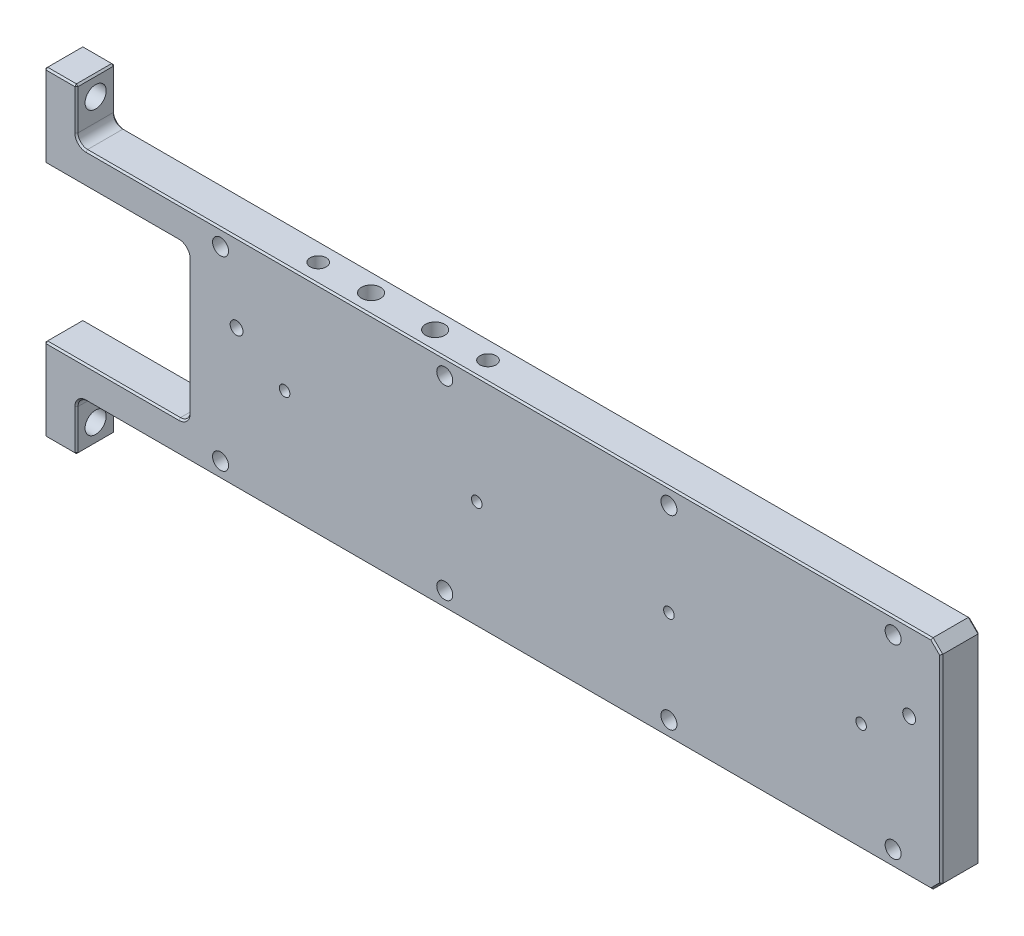
SolidWorks part; units mm, degrees
material "#45(1.1191)"
ref_plane "前视基准面" through (0, 0, 0) normal (0, 0, 1) x (1, 0, 0)
ref_plane "上视基准面" through (0, 0, 0) normal (0, 1, 0) x (1, 0, 0)
ref_plane "右视基准面" through (0, 0, 0) normal (1, 0, 0) x (0, 0, -1)
sketch "草图1" plane through (0, 0, 0) normal (0, 0, 1) x (1, 0, 0)
  line L1 (-140, -34) -> (140, -34)
  line L2 (-140, -34) -> (-140, 34)
  line L3 (-140, 34) -> (140, 34)
  line L4 (140, -34) -> (140, 34)
  line L5 (-140, -34) -> (140, 34) construction
  line L6 (-140, 34) -> (140, -34) construction
  point P0 (0, 0)
  dimension "D1" = 280
  dimension "D2" = 68
extrude "凸台-拉伸1" add sketch "草图1" along normal mid plane 12
sketch "草图2" plane through (0, 0, -6) normal (0, 0, -1) x (-1, 0, 0)
  line L0 (-140, 0) -> (140, 0) construction
  line L1 (95, -24) -> (140, -24)
  line L2 (95, -24) -> (95, 24)
  line L3 (95, 24) -> (140, 24)
  line L4 (140, -24) -> (140, 24)
  line L5 (-140, -34) -> (-140, 34) construction
  line L6 (140, 34) -> (140, -34) construction
  dimension "D1" = 48
  dimension "D2" = 45
extrude "切除-拉伸1" cut sketch "草图2" against normal blind 25
fillet "圆角1" radius 3 2 edges at (-95, -24, 0) (-95, 24, 0)
sketch "草图3" plane through (-140, 0, 0) normal (-1, 0, 0) x (0, 0, 1)
  line L0 (6, 0) -> (-6, 0) construction
  line L1 (6, 21) -> (6, -21) construction
  line L2 (-6, 21) -> (-6, -21) construction
  line L3 (0, 34) -> (0, -34) construction
  line L4 (6, 34) -> (-6, 34) construction
  line L5 (6, -34) -> (-6, -34) construction
  line L6 (-6, -24) -> (-6, -34) construction
  line L7 (6, -34) -> (-6, -34)
  line L8 (6, -34) -> (6, -50)
  line L9 (6, -50) -> (-6, -50)
  line L10 (-6, -34) -> (-6, -50)
  line L11 (-6, 34) -> (-6, 50)
  line L12 (6, 50) -> (-6, 50)
  line L13 (6, 34) -> (6, 50)
  line L14 (6, 34) -> (-6, 34)
  dimension "D1" = 16
extrude "凸台-拉伸2" add sketch "草图3" against normal blind 10
fillet "圆角2" radius 3 2 edges at (-130, 34, 0) (-130, -34, 0)
sketch "草图4" plane through (-130, 0, 0) normal (1, 0, 0) x (0, 0, -1)
  line L0 (0, -50) -> (0, 50) construction
  line L1 (6, -50) -> (-6, -50) construction
  line L2 (-6, 50) -> (6, 50) construction
  line L4 (-6, 0) -> (6, 0) construction
  line L5 (-6, -34) -> (-6, 34) construction
  line L6 (6, -34) -> (6, 34) construction
  point P0 (0, -44)
  point P18 (0, 44)
  dimension "D1" = 6
hole_wizard "M6 间隙孔1" positions "草图4" profile "草图5" hole size "M6" standard "ISO" end condition through all
sketch "草图5" plane through (-130, -44, 0) normal (0, 1, 0) x (0, 0, -1)
  line L0 (0, 0) -> (0, 10)
  line L1 (0, 10) -> (3.3, 10)
  line L2 (3.3, 10) -> (3.3, 0)
  line L5 (3.3, 0) -> (0, 0)
  line L11 (0, -6.35) -> (0, 107.95) construction
  dimension "通孔孔直径" = 6.6
  dimension "通孔孔深度" = 10
sketch "草图6" plane through (-140, 0, 0) normal (-1, 0, 0) x (0, 0, 1)
  line L0 (6, 0) -> (-6, 0) construction
  line L1 (6, 21) -> (6, -21) construction
  line L2 (-6, 21) -> (-6, -21) construction
  line L4 (0, 50) -> (0, -50) construction
  line L5 (6, 50) -> (-6, 50) construction
  line L6 (-6, -50) -> (6, -50) construction
  point P0 (0, 32.5)
  point P20 (0, -32.5)
  dimension "D1" = 65
hole_wizard "Ø6.0mm 暗销孔1" positions "草图6" profile "草图7" hole size "Ø6.0" standard "ISO"
sketch "草图7" plane through (-140, 32.5, 0) normal (0, 1, 0) x (0, 0, 1)
  line L0 (0, 0) -> (0, 11.8026)
  line L1 (0, 11.8026) -> (3, 10)
  line L2 (3, 10) -> (3, 0)
  line L5 (3, 0) -> (0, 0)
  line L10 (0, 11.8026) -> (-3, 10) construction
  line L11 (0, -6.35) -> (0, 107.95) construction
  dimension "孔直径" = 6
  dimension "孔深度" = 10
  dimension "导头角度" = 118
chamfer "倒角1" distance 3 angle 45 2 edges at (140, 34, 0) (140, -34, 0)
chamfer "倒角2" distance 0.5 angle 45 42 edges at (-119, 24, -6) (-119, 24, 6) (-119, -24, 6) (-119, -24, -6) (-95.8787, 23.1213, 6) (-95.8787, 23.1213, -6) (-95.8787, -23.1213, 6) (-95.8787, -23.1213, -6) (-95, 0, -6) (-95, 0, 6) (-135, -50, 6) (-130, -50, 0) (-135, -50, -6) (-140, -50, 0) (-140, -37, 6) (-140, -37, -6) (-140, -24, 0) (-135, 50, -6) (-130, 50, 0) (-135, 50, 6) (-140, 50, 0) (-140, 37, 6) (-140, 37, -6) (-140, 24, 0) (-130, 43.5, 6) (-130, -43.5, 6) (-129.1213, 34.8787, -6) (-129.1213, 34.8787, 6) (-129.1213, -34.8787, 6) (-129.1213, -34.8787, -6) (5, 34, 6) (5, 34, -6) (138.5, 32.5, 6) (138.5, 32.5, -6) (140, 0, -6) (140, 0, 6) (138.5, -32.5, 6) (138.5, -32.5, -6) (5, -34, -6) (5, -34, 6) (-130, 43.5, -6) (-130, -43.5, -6)
sketch "草图16" plane through (0, 0, -6) normal (0, 0, -1) x (-1, 0, 0)
  point P0 (-125, 29)
  point P3 (-125, -29)
  point P6 (-55, 29)
  point P9 (-55, -29)
  point P12 (15, 29)
  point P15 (15, -29)
  point P18 (85, 29)
  point P21 (85, -29)
hole_wizard "M6 螺纹孔3" positions "草图16" profile "草图17" tap size "M6" standard "ISO" end condition through all
sketch "草图17" plane through (125, 29, -6) normal (1, 0, 0) x (0, 1, 0)
  line L0 (0, 0) -> (0, 12)
  line L1 (0, 12) -> (2.5, 12)
  line L2 (2.5, 12) -> (2.5, 0)
  line L5 (2.5, 0) -> (0, 0)
  line L11 (0, -6.35) -> (0, 107.95) construction
  dimension "通孔螺纹孔钻头直径" = 5
  dimension "通孔螺纹孔钻头深度" = 12
cosmetic thread "孔螺蚊线14" parameters "D2"=6
cosmetic thread "孔螺蚊线15" parameters "D2"=6
cosmetic thread "孔螺蚊线16" parameters "D2"=6
cosmetic thread "孔螺蚊线17" parameters "D2"=6
cosmetic thread "孔螺蚊线18" parameters "D2"=6
cosmetic thread "孔螺蚊线19" parameters "D2"=6
cosmetic thread "孔螺蚊线22" parameters "D2"=6
cosmetic thread "孔螺蚊线23" parameters "D2"=6
sketch "草图18" plane through (0, 34, 0) normal (0, 1, 0) x (1, 0, 0)
  point P0 (-24, 0)
  point P3 (-44, 0)
hole_wizard "Ø6.0mm 暗销孔2" positions "草图18" profile "草图19" hole size "Ø6.0" standard "ISO"
sketch "草图19" plane through (-24, 34, 0) normal (1, 0, 0) x (0, 0, 1)
  line L0 (0, 0) -> (0, 7.8026)
  line L1 (0, 7.8026) -> (3, 6)
  line L2 (3, 6) -> (3, 0)
  line L5 (3, 0) -> (0, 0)
  line L10 (0, 7.8026) -> (-3, 6) construction
  line L11 (0, -6.35) -> (0, 107.95) construction
  dimension "孔直径" = 6
  dimension "孔深度" = 6
  dimension "导头角度" = 118
sketch "草图20" plane through (0, 34, 0) normal (0, 1, 0) x (1, 0, 0)
  point P0 (-7.5, 0)
  point P3 (-60.5, 0)
hole_wizard "M6 螺纹孔4" positions "草图20" profile "草图21" tap size "M6" standard "ISO"
sketch "草图21" plane through (-7.5, 34, 0) normal (1, 0, 0) x (0, 0, 1)
  line L0 (0, 0) -> (0, 16.5022)
  line L1 (0, 16.5022) -> (2.5, 15)
  line L2 (2.5, 15) -> (2.5, 0)
  line L5 (2.5, 0) -> (0, 0)
  line L10 (0, 16.5022) -> (-2.5, 15) construction
  line L11 (0, -6.35) -> (0, 107.95) construction
  dimension "螺纹孔钻头直径" = 5
  dimension "螺纹孔钻头深度" = 15
  dimension "导头角度" = 118
cosmetic thread "孔螺蚊线24" parameters "D1"=12, "D2"=6
cosmetic thread "孔螺蚊线25" parameters "D1"=12, "D2"=6
hole_wizard "M4 螺纹孔1" positions "草图23" profile "草图22" tap size "M4" standard "ISO" end condition through all
sketch "草图23" plane through (0, 0, 6) normal (0, 0, 1) x (1, 0, 0)
  circle A0 centre (115, 0) radius 2.25 construction
  circle A1 centre (55, 0) radius 2.25 construction
  circle A2 centre (-65, 0) radius 2.25 construction
  circle A3 centre (-5, 0) radius 2.25 construction
  point P1 (115, 0)
  point P4 (55, 0)
  point P7 (-65, 0)
  point P10 (-5, 0)
sketch "草图22" plane through (115, 0, 6) normal (1, 0, 0) x (0, -1, 0)
  line L0 (0, 0) -> (0, 12)
  line L1 (0, 12) -> (1.65, 12)
  line L2 (1.65, 12) -> (1.65, 0)
  line L5 (1.65, 0) -> (0, 0)
  line L11 (0, -6.35) -> (0, 107.95) construction
  dimension "通孔螺纹孔钻头直径" = 3.3
  dimension "通孔螺纹孔钻头深度" = 12
cosmetic thread "孔螺蚊线26" parameters "D2"=4
cosmetic thread "孔螺蚊线27" parameters "D2"=4
cosmetic thread "孔螺蚊线28" parameters "D2"=4
cosmetic thread "孔螺蚊线29" parameters "D2"=4
hole_wizard "Ø4.0 mm 暗销孔1" positions "草图25" profile "草图24" hole size "Ø4.0" standard "ISO"
sketch "草图25" plane through (0, 0, 6) normal (0, 0, 1) x (1, 0, 0)
  line L0 (135, 7.5) -> (-85, 7.5) construction
  point P1 (-80, 9.5)
  point P5 (130, 9.5)
  dimension "D1" = 2
  dimension "D2" = 5.3852
  dimension "D3" = 2
  dimension "D4" = 5.3852
sketch "草图24" plane through (-80, 9.5, 6) normal (1, 0, 0) x (0, -1, 0)
  line L0 (0, 0) -> (0, 5)
  line L1 (0, 5) -> (2, 5)
  line L2 (2, 5) -> (2, 0)
  line L5 (2, 0) -> (0, 0)
  line L10 (0, 5) -> (-2, 5) construction
  line L11 (0, -6.35) -> (0, 107.95) construction
  dimension "孔直径" = 4
  dimension "孔深度" = 5
  dimension "导头角度" = 180
